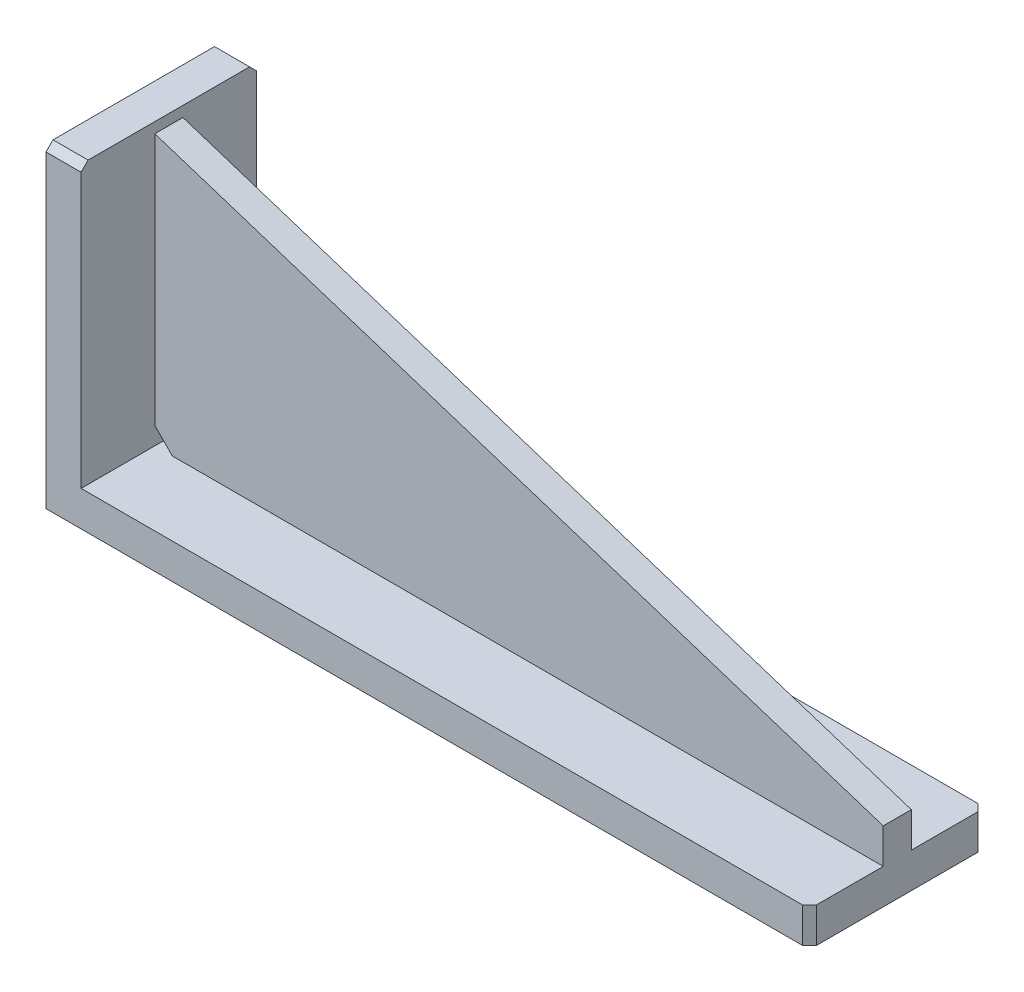
from build123d import *

# Parameters (mm, degrees)
EXTRUDE_1_DEPTH = 25
EXTRUDE_2_DEPTH = 4
CHAMFER_1_SIZE  = 2


with BuildPart() as part:
    # 草图1 → 凸台-拉伸1 (new, symmetric)
    with BuildSketch(Plane.XY):
        Polygon((0, 0), (217.5, 0), (217.5, 10), (10, 10), (10, 90), (0, 90), align=None)
    extrude(amount=EXTRUDE_1_DEPTH, both=True)

    # 草图2 → 凸台-拉伸2 (add, symmetric)
    with BuildSketch(Plane.XY):
        Polygon((10, 87), (217.5, 20), (217.5, 10), (15, 10), (10, 15), align=None)
    extrude(amount=EXTRUDE_2_DEPTH, both=True)

    # 倒角1
    chamfer_1_edges = [part.edges().sort_by_distance(p)[0] for p in [
        (217.5, 5, 25),
        (5, 90, 25),
        (5, 90, -25),
        (217.5, 5, -25),
    ]]
    chamfer(chamfer_1_edges, length=CHAMFER_1_SIZE)


solid = part.part
